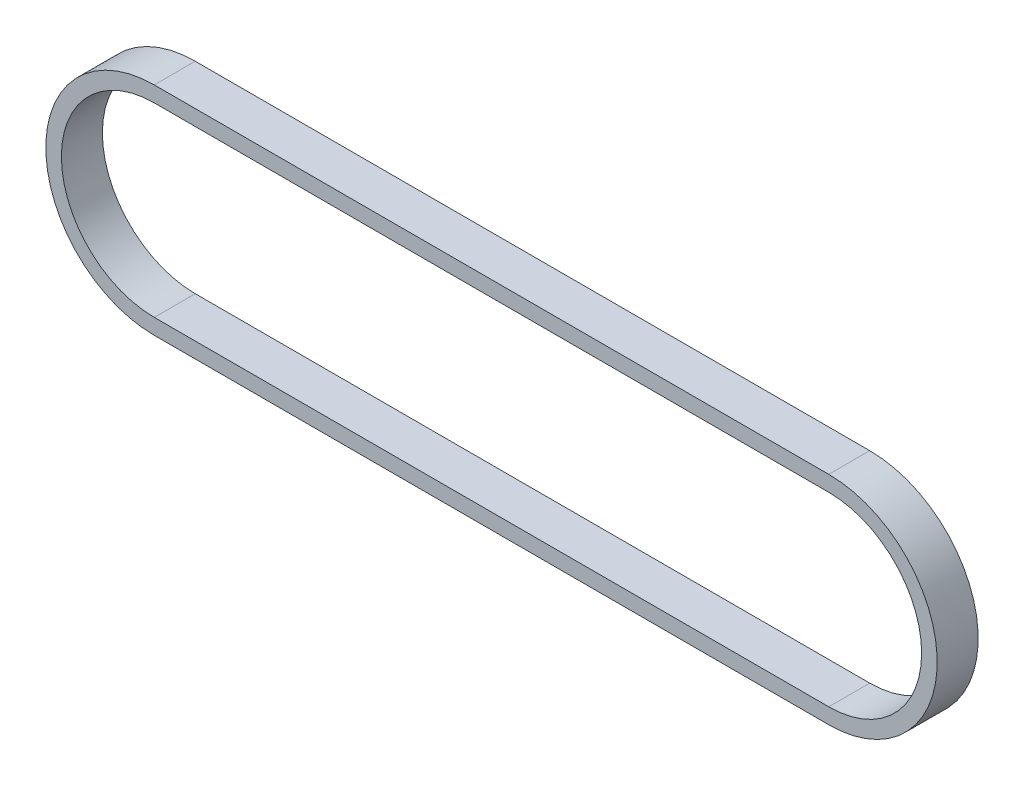
SolidWorks part; units mm, degrees
ref_plane "Front Plane" through (0, 0, 0) normal (0, 0, 1) x (1, 0, 0)
ref_plane "Top Plane" through (0, 0, 0) normal (0, 1, 0) x (1, 0, 0)
ref_plane "Right Plane" through (0, 0, 0) normal (1, 0, 0) x (0, 0, -1)
sketch "Sketch2" plane through (0, 0, 0) normal (0, 0, 1) x (1, 0, 0)
  line L0 (5.5, 0) -> (-5.5, 0) construction
  line L1 (0, 20.9) -> (-130, 20.9)
  line L2 (0, -20.9) -> (-130, -20.9)
  arc A0 (0, -20.9) -> (0, 20.9) centre (0, 0) ccw
  arc A1 (-130, 20.9) -> (-130, -20.9) centre (-130, 0) ccw
  dimension "D1" = 41.8
  dimension "D2" = 41.8
  dimension "D3" = 130
extrude "Boss-Extrude1" add sketch "Sketch2" along normal blind 7.9
shell "Shell1" thickness 3
